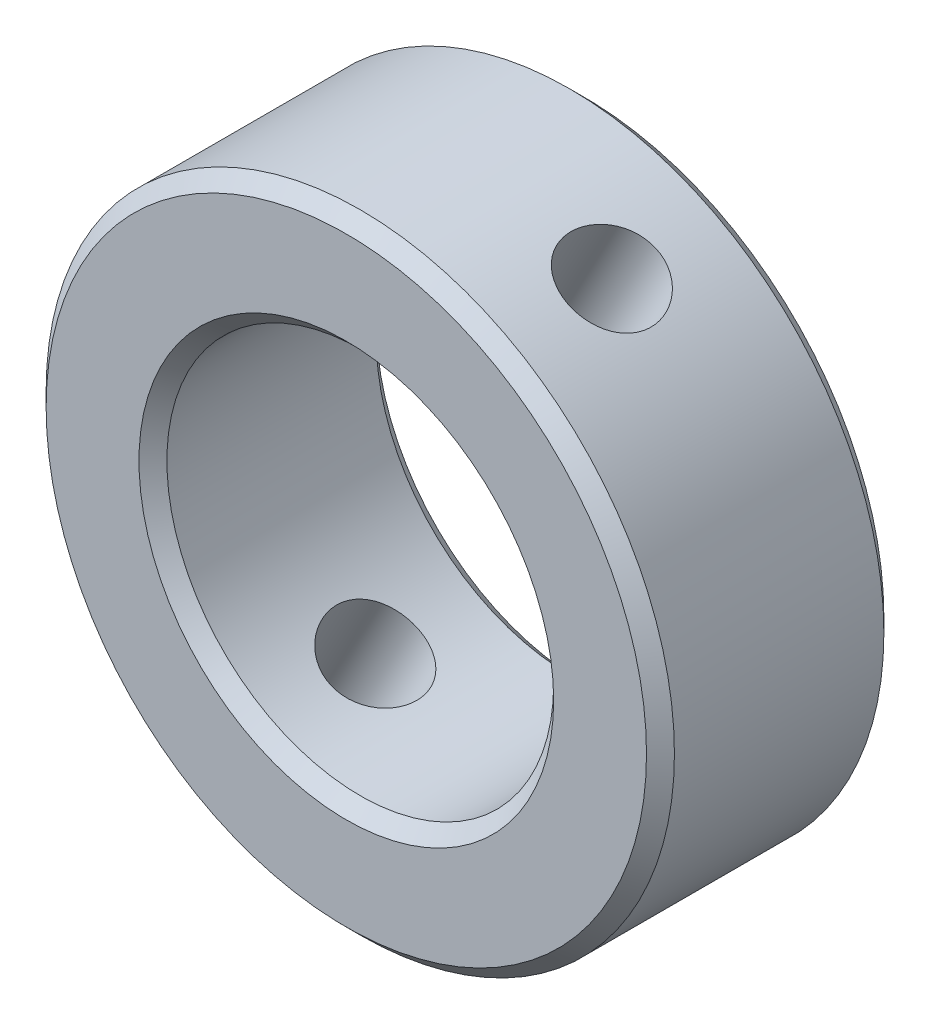
from build123d import *

# Parameters (mm, degrees)
SKETCH1_R                  = 45
SKETCH1_R_2                = 27.7
BOSS_EXTRUDE1_DEPTH        = 34
F_13_0_13_DIAMETER_HOLE1_D = 13
CHAMFER1_SIZE              = 2


with BuildPart() as part:
    # Sketch1 → Boss-Extrude1 (new body)
    with BuildSketch(Plane.XY):
        Circle(SKETCH1_R)
        Circle(SKETCH1_R_2, mode=Mode.SUBTRACT)
    extrude(amount=BOSS_EXTRUDE1_DEPTH)

    # Ø13.0 (13) Diameter Hole1 (through all)
    with Locations(Plane(origin=(21.131064714, 39.730065493, 17), x_dir=(0.882890344282, -0.469579215865, 0), z_dir=(0.469579215865, 0.882890344282, 0))):
        with Locations((0, 0)):
            Hole(F_13_0_13_DIAMETER_HOLE1_D / 2)

    # Chamfer1
    chamfer1_edges = [part.edges().sort_by_distance(p)[0] for p in [
        (-45, 0, 0),
        (-45, 0, 34),
        (-27.7, 0, 0),
        (-27.7, 0, 34),
    ]]
    chamfer(chamfer1_edges, length=CHAMFER1_SIZE)


solid = part.part
